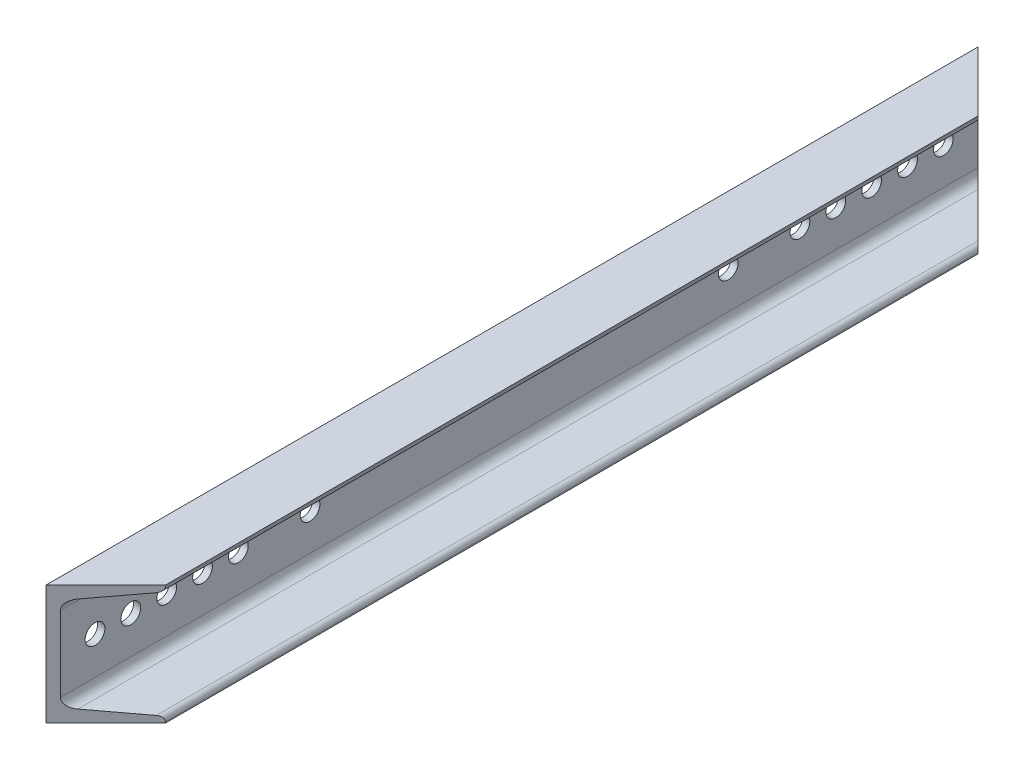
from build123d import *

# Parameters (mm, degrees)
BOSS_EXTRUDE1_DEPTH = 1000
CUT_EXTRUDE4_DEPTH  = 100
SKETCH6_R           = 8.25
CUT_EXTRUDE5_DEPTH  = 100


with BuildPart() as part:
    # Sketch1 → Boss-Extrude1 (new body)
    with BuildSketch(Plane.XY):
        with BuildLine():
            Line((0, 0), (0, -100))
            Line((0, -100), (50, -100))
            Line((50, -100), (50, -98.925311188))
            ThreePointArc((50, -98.925311188), (48.896193111, -95.973045557), (46.126278954, -94.469104878))
            Line((46.126278954, -94.469104878), (13.317028642, -89.858065454))
            ThreePointArc((13.317028642, -89.858065454), (8.084968568, -87.017288616), (6, -81.440786869))
            Line((6, -81.440786869), (6, -18.559213131))
            ThreePointArc((6, -18.559213131), (8.084968568, -12.982711384), (13.317028642, -10.141934546))
            Line((13.317028642, -10.141934546), (46.126278954, -5.530895122))
            ThreePointArc((46.126278954, -5.530895122), (48.896193111, -4.026954443), (50, -1.074688812))
            Line((50, -1.074688812), (50, 0))
            Line((50, 0), (0, 0))
        make_face()
    extrude(amount=BOSS_EXTRUDE1_DEPTH)

    # Sketch5 → Cut-Extrude4 (cut)
    with BuildSketch(Plane(origin=(0, 0, 0), x_dir=(1, 0, 0), z_dir=(0, 1, 0))):
        Polygon((0, -111.192266245), (155.007948876, -266.200215121), (155.007948876, 58.518788552), (-221.01044115, 43.925946333), align=None)
        Polygon((197.398911987, -693.793354258), (279.115957405, -1211.070261728), (0, -1168.351944778), (-115.400263834, -952.431807993), (0, -891.192266245), align=None)
    extrude(amount=-CUT_EXTRUDE4_DEPTH, mode=Mode.SUBTRACT)

    # Sketch6 → Cut-Extrude5 (cut)
    with BuildSketch(Plane.ZY):
        with Locations(Location((146.192266245, -50, 0), (0, 0, 270))):
            Circle(SKETCH6_R)
        with Locations(Location((176.192266245, -50, 0), (0, 0, 270))):
            Circle(SKETCH6_R)
        with Locations(Location((206.192266245, -50, 0), (0, 0, 270))):
            Circle(SKETCH6_R)
        with Locations(Location((236.192266245, -50, 0), (0, 0, 270))):
            Circle(SKETCH6_R)
        with Locations(Location((266.192266245, -50, 0), (0, 0, 270))):
            Circle(SKETCH6_R)
        with Locations(Location((326.192266245, -50, 0), (0, 0, 270))):
            Circle(SKETCH6_R)
        with Locations(Location((676.192266245, -50, 0), (0, 0, 270))):
            Circle(SKETCH6_R)
        with Locations(Location((736.192266245, -50, 0), (0, 0, 270))):
            Circle(SKETCH6_R)
        with Locations(Location((766.192266245, -50, 0), (0, 0, 270))):
            Circle(SKETCH6_R)
        with Locations(Location((796.192266245, -50, 0), (0, 0, 270))):
            Circle(SKETCH6_R)
        with Locations(Location((826.192266245, -50, 0), (0, 0, 270))):
            Circle(SKETCH6_R)
        with Locations(Location((856.192266245, -50, 0), (0, 0, 270))):
            Circle(SKETCH6_R)
    extrude(amount=-CUT_EXTRUDE5_DEPTH, mode=Mode.SUBTRACT)


solid = part.part
